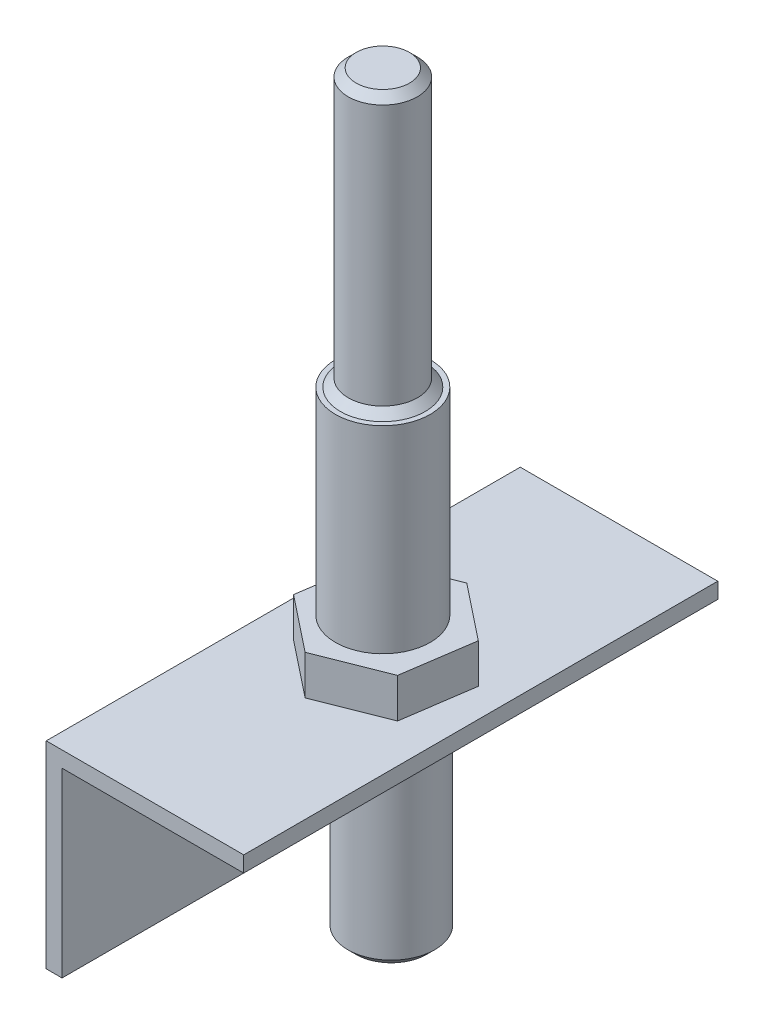
from build123d import *

# Parameters (mm, degrees)
EXTRUDE_THIN1_DEPTH = 60
BOSS_EXTRUDE2_DEPTH = 5
SKETCH4_R           = 5.5
BOSS_EXTRUDE3_DEPTH = 25
SKETCH5_R           = 6
BOSS_EXTRUDE4_DEPTH = 25
SKETCH6_R           = 4.372501997
BOSS_EXTRUDE5_DEPTH = 35
CHAMFER1_SIZE       = 1


with BuildPart() as part:
    # Sketch2 → Extrude-Thin1 (new body)
    with BuildSketch(Plane.XY):
        Polygon((0, 0), (0, 25), (25, 25), (25, 23), (2, 23), (2, 0), align=None)
    extrude(amount=EXTRUDE_THIN1_DEPTH)

    # Sketch3 → Boss-Extrude2 (add, symmetric)
    with BuildSketch(Plane(origin=(0, 25, 0), x_dir=(1, 0, 0), z_dir=(0, 1, 0))):
        Polygon((11.684931341, -38.911131142), (20.059731616, -35.594448438), (21.374800275, -26.683317296), (14.315068659, -21.088868858), (5.940268384, -24.405551562), (4.625199725, -33.316682704), align=None)
    extrude(amount=BOSS_EXTRUDE2_DEPTH, both=True)

    # Sketch4 → Boss-Extrude3 (add)
    with BuildSketch(Plane(origin=(0, 20, 0), x_dir=(-1, 0, 0), z_dir=(0, -1, 0))):
        with Locations(Location((-13, -29.319447598, 0), (0, 0, 270))):
            Circle(SKETCH4_R)
    extrude(amount=BOSS_EXTRUDE3_DEPTH)

    # Sketch5 → Boss-Extrude4 (add)
    with BuildSketch(Plane(origin=(0, 30, 0), x_dir=(1, 0, 0), z_dir=(0, 1, 0))):
        with Locations(Location((12.519179725, -29.915081058, 0), (0, 0, 270))):
            Circle(SKETCH5_R)
    extrude(amount=BOSS_EXTRUDE4_DEPTH)

    # Sketch6 → Boss-Extrude5 (add)
    with BuildSketch(Plane(origin=(0, 55, 0), x_dir=(1, 0, 0), z_dir=(0, 1, 0))):
        with Locations(Location((12.519179725, -29.915081058, 0), (0, 0, 270))):
            Circle(SKETCH6_R)
    extrude(amount=BOSS_EXTRUDE5_DEPTH)

    # Chamfer1
    chamfer1_edges = [part.edges().sort_by_distance(p)[0] for p in [
        (13, -5, 23.819447598),
        (12.519179725, 55, 25.542579061),
        (12.519179725, 90, 25.542579061),
    ]]
    chamfer(chamfer1_edges, length=CHAMFER1_SIZE)


solid = part.part
